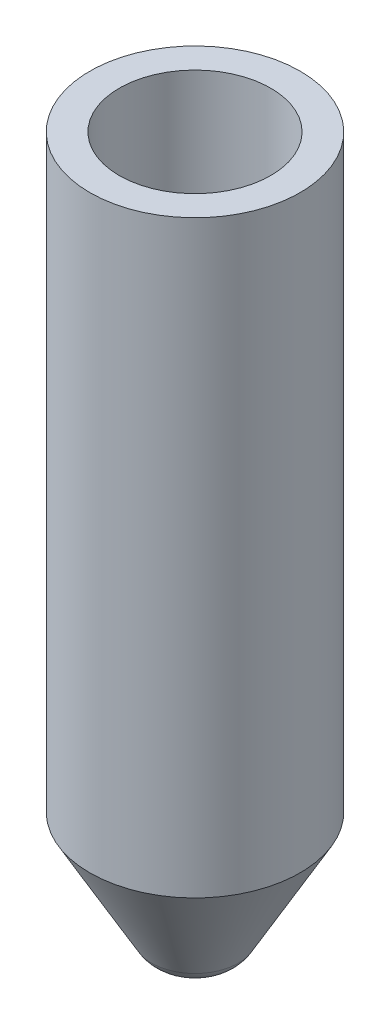
SolidWorks part; units mm, degrees
ref_plane "Front Plane" through (0, 0, 0) normal (0, 0, 1) x (1, 0, 0)
ref_plane "Top Plane" through (0, 0, 0) normal (0, 1, 0) x (1, 0, 0)
ref_plane "Right Plane" through (0, 0, 0) normal (1, 0, 0) x (0, 0, -1)
sketch "Sketch2" plane through (0, 0, 0) normal (0, 0, 1) x (1, 0, 0)
  line L1 (0, 1700) -> (250, 1700)
  line L2 (250, 1700) -> (250, 300)
  line L4 (0, 0) -> (0, 517.7773) construction
  line L6 (0, 1700) -> (0, 0)
  line L7 (0, 0) -> (80, 0)
  line L8 (80, 0) -> (250, 300)
  dimension "D4" = 1400
  dimension "D1" = 250
  dimension "D2" = 1700
  dimension "D3" = 80
revolve "Revolve1" add sketch "Sketch2" angle 360 about L4
fillet "Fillet1" radius 80 1 edges at (0, 0, -80)
shell "Shell1" thickness 70
